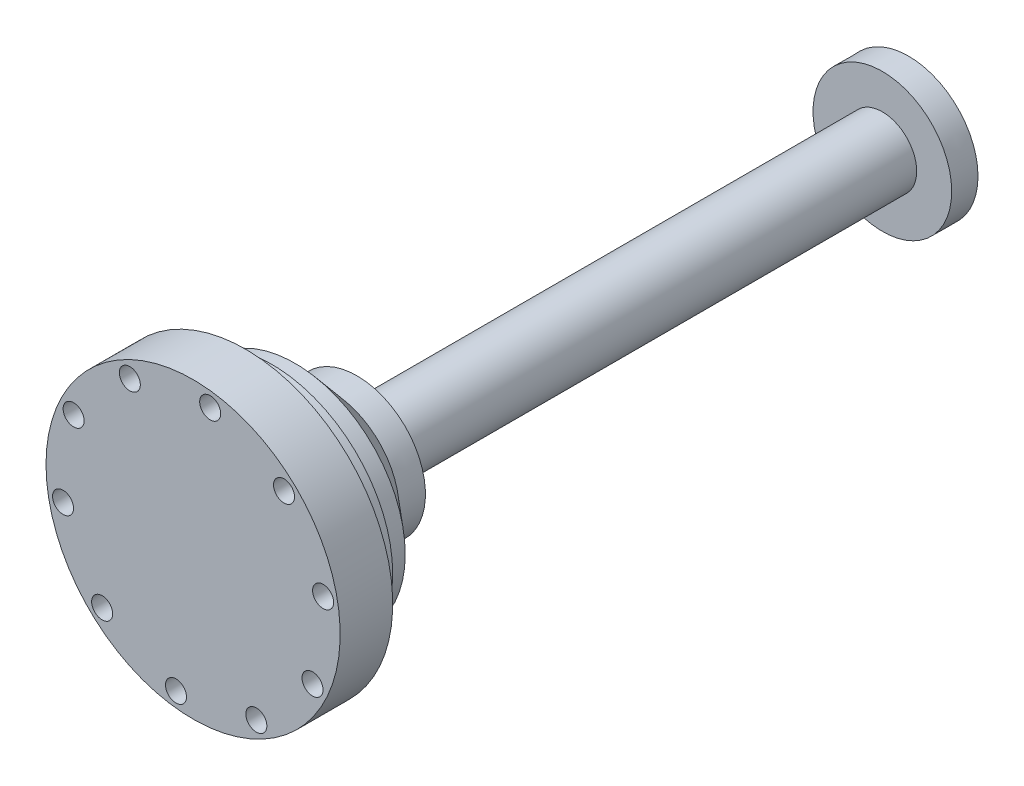
from build123d import *

# Parameters (mm, degrees)
SKETCH5_W           = 13.145964729
SKETCH5_H           = 100
SKETCH6_R           = 28
BOSS_EXTRUDE1_DEPTH = 10
SKETCH7_R           = 2
CUT_EXTRUDE1_DEPTH  = 10
CIRPATTERN1_COUNT   = 10


with BuildPart() as part:
    # Sketch4 → Revolve1 (revolve)
    with BuildSketch(Plane(origin=(20, 0, 0), x_dir=(0, -1, 0), z_dir=(-1, 0, 0)), mode=Mode.PRIVATE) as revolve1_sk:
        Polygon((-76.830512452, 0), (-76.830512452, -4.383431838), (-68.830512452, -11.214554774), (-69.034523253, -121.214554774), (-55.830512452, -121.214554774), (-55.830512452, 15), (-78.802692797, 15), (-78.830512452, 0), align=None)
    revolve(revolve1_sk.sketch.rotate(Axis((20, 55.830512452, 15), (0, 0, -1)), 90), axis=Axis((20, 55.830512452, 15), (0, 0, -1)))

    # Sketch5 → Cut-Revolve1 (revolve, cut)
    with BuildSketch(Plane(origin=(20, 0, 0), x_dir=(0, -1, 0), z_dir=(-1, 0, 0)), mode=Mode.PRIVATE) as cut_revolve1_sk:
        with Locations((-42.728507052, -66.214554774)):
            Rectangle(SKETCH5_W, SKETCH5_H)
    revolve(cut_revolve1_sk.sketch.rotate(Axis((20, 55.830512452, -11.214554774), (0, 0, -1)), 270), axis=Axis((20, 55.830512452, -11.214554774), (0, 0, -1)), mode=Mode.SUBTRACT)

    # Sketch6 → Boss-Extrude1 (add)
    with BuildSketch(Plane(origin=(0, 0, 15), x_dir=(-1, 0, 0), z_dir=(0, 0, -1))):
        with Locations((-20, 55.830512452)):
            Circle(SKETCH6_R)
    extrude(amount=BOSS_EXTRUDE1_DEPTH)

    # Sketch7 → Cut-Extrude1 (cut)
    with BuildSketch(Plane(origin=(0, 0, 5), x_dir=(-1, 0, 0), z_dir=(0, 0, -1))):
        with Locations((4.75295766, 51.209902338)):
            Circle(SKETCH7_R)
    cut_extrude1 = extrude(amount=-CUT_EXTRUDE1_DEPTH, mode=Mode.SUBTRACT)

    # CirPattern1: Cut-Extrude1 ×10 about axis
    cirpattern1_axis = Axis((20, 55.830512452, 0), (0, 0, 1))
    for i in range(1, CIRPATTERN1_COUNT):
        add(cut_extrude1.rotate(cirpattern1_axis, i * 360 / CIRPATTERN1_COUNT), mode=Mode.SUBTRACT)


solid = part.part
